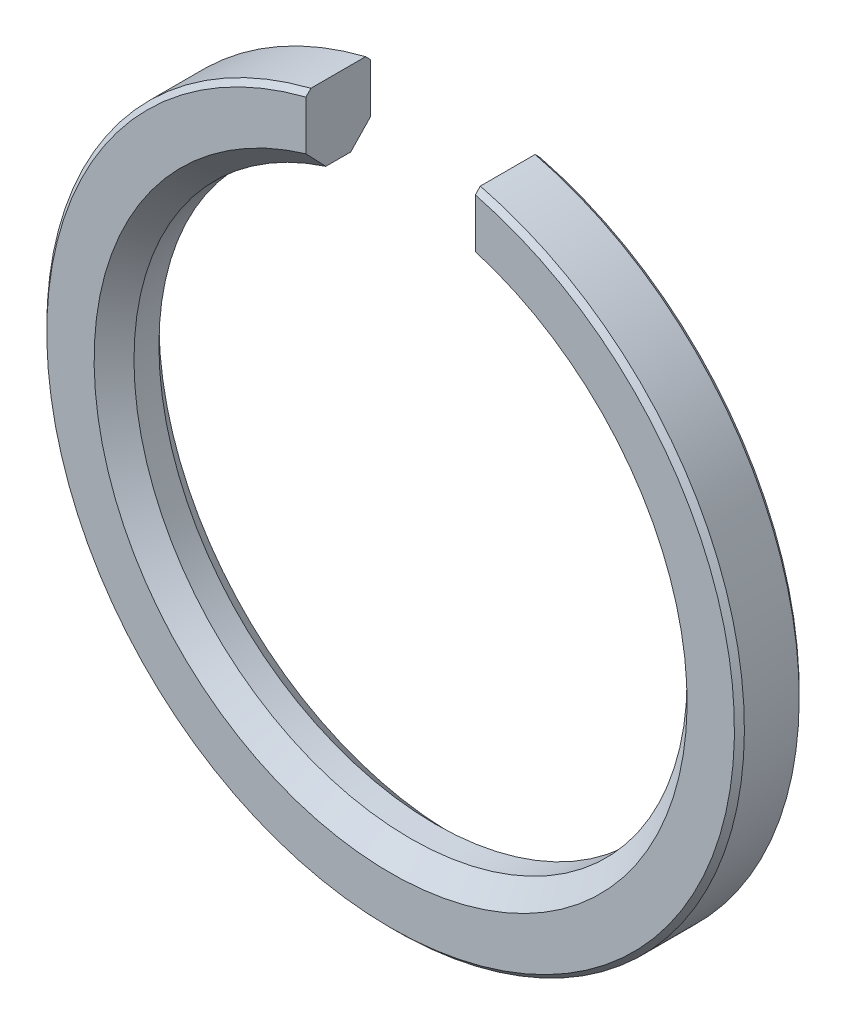
from build123d import *

# Parameters (mm, degrees)
SKETCH1_R           = 35
SKETCH1_R_2         = 27.75
BOSS_EXTRUDE1_DEPTH = 6.5
CUT_EXTRUDE1_DEPTH  = 50.922439844
CHAMFER1_SIZE       = 2
CHAMFER2_SIZE       = 0.5


with BuildPart() as part:
    # Sketch1 → Boss-Extrude1 (new body)
    with BuildSketch(Plane.XY):
        with Locations(Location((0, 0, 0), (0, 0, 180))):
            Circle(SKETCH1_R)
        with Locations(Location((0, 0, 0), (0, 0, 180))):
            Circle(SKETCH1_R_2, mode=Mode.SUBTRACT)
    extrude(amount=BOSS_EXTRUDE1_DEPTH)

    # Sketch2 → Cut-Extrude1 (cut, through all)
    with BuildSketch(Plane.XY.offset(6.5)):
        Polygon((0, 0), (8.5, 0), (8.5, 53.904694855), (-8.5, 53.904694855), (-8.5, 0), align=None)
    extrude(amount=-CUT_EXTRUDE1_DEPTH, mode=Mode.SUBTRACT)

    # Chamfer1
    chamfer1_edges = [part.edges().sort_by_distance(p)[0] for p in [
        (0, -27.75, 0),
        (0, -27.75, 6.5),
    ]]
    chamfer(chamfer1_edges, length=CHAMFER1_SIZE)

    # Chamfer2
    chamfer2_edges = [part.edges().sort_by_distance(p)[0] for p in [
        (0, -35, 6.5),
        (0, -35, 0),
    ]]
    chamfer(chamfer2_edges, length=CHAMFER2_SIZE)


solid = part.part
